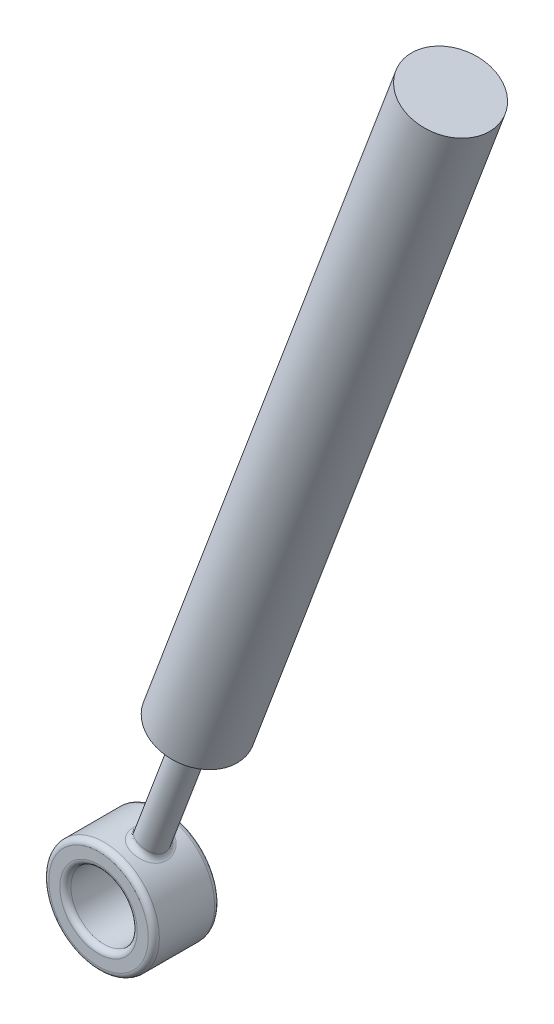
from build123d import *

# Parameters (mm, degrees)
BOSS_EXTRUDE1_START      = -260
BOSS_EXTRUDE1_DEPTH      = 260
BOSS_EXTRUDE4_DEPTH      = 24
BOSS_EXTRUDE5_REACH      = 2447.334
BOSS_EXTRUDE5_END_RADIUS = 20
SKETCH5_R                = 5
FILLET1_R                = 2
FILLET2_R                = 2
CHAMFER2_SIZE            = 1


with BuildPart() as part:
    # Sketch1 → Boss-Extrude1 (new body)
    with BuildSketch(Plane(origin=(83.573308801, 222.892709782, 0), x_dir=(0.9363450005078556, -0.3510812441927706, 0), z_dir=(-0.3510812441927706, -0.9363450005078556, 0)).offset(BOSS_EXTRUDE1_START)):
        with BuildLine():
            ThreePointArc((546.192823225, 2320.014515708), (561.248526003, 2335.070218486), (546.192823225, 2350.125921264))
            ThreePointArc((546.192823225, 2350.125921264), (531.137120447, 2335.070218486), (546.192823225, 2320.014515708))
        make_face()
    extrude(amount=BOSS_EXTRUDE1_DEPTH)



with BuildPart() as body_2:
    # Sketch6 → Boss-Extrude4 (new body)
    with BuildSketch(Plane(origin=(0, 0, 2323.070218486), x_dir=(-1, 0, 0), z_dir=(0, 0, -1))):
        with BuildLine():
            ThreePointArc((-589.676062924, -40.026603584), (-563.92753803, -51.73187871), (-552.222262904, -25.983353816))
            ThreePointArc((-552.222262904, -25.983353816), (-577.970787798, -14.27807869), (-589.676062924, -40.026603584))
        make_face()
        with BuildLine():
            ThreePointArc((-582.18530292, -37.21795363), (-566.736188003, -44.241118713), (-559.713022893, -28.792003808))
            ThreePointArc((-559.713022893, -28.792003808), (-575.162137825, -21.768838687), (-582.18530292, -37.21795363))
        make_face(mode=Mode.SUBTRACT)
    extrude(amount=-BOSS_EXTRUDE4_DEPTH)


with BuildPart() as part_1:
    add(part.part)

    add(body_2.part)  # Boss-Extrude5 merges body 2
    # Boss-Extrude5: up to this cylinder (the profile starts outside it)
    boss_extrude5_end = Plane(origin=(570.949162914, -33.0049787, 2335.070218), z_dir=(0, 0, -1)) * Cylinder(BOSS_EXTRUDE5_END_RADIUS, 4935.668, mode=Mode.PRIVATE)
    # Sketch5 → Boss-Extrude5 (add, up to the surface)
    with BuildSketch(Plane(origin=(83.573308801, 222.892709782, 0), x_dir=(0.9363450005078556, -0.3510812441927706, 0), z_dir=(-0.3510812441927706, -0.9363450005078556, 0)), mode=Mode.PRIVATE) as boss_extrude5_sk1:
        with Locations(Location((546.192823225, 2335.070218486, 0), (0, 0, 180))):
            Circle(SKETCH5_R)
    boss_extrude5_tool1 = extrude(boss_extrude5_sk1.sketch, amount=BOSS_EXTRUDE5_REACH, mode=Mode.PRIVATE) - boss_extrude5_end
    add(boss_extrude5_tool1.solids().sort_by_distance((594.998228, 31.134654, 2335.070218))[0])

    # Fillet1
    fillet1_edges = [part_1.edges().sort_by_distance(p)[0] for p in [
        (582.429546976, -16.628141955, 2335.070218486),
    ]]
    fillet(fillet1_edges, radius=FILLET1_R)

    # Fillet2
    fillet2_edges = [part_1.edges().sort_by_distance(p)[0] for p in [
        (559.713022908, -28.79200377, 2347.070218486),
        (589.676062924, -40.026603584, 2347.070218486),
        (559.713022908, -28.79200377, 2323.070218486),
        (589.676062924, -40.026603584, 2323.070218486),
    ]]
    fillet(fillet2_edges, radius=FILLET2_R)

    # Chamfer2
    chamfer2_edges = [part_1.edges().sort_by_distance(p)[0] for p in [
        (599.679953144, 29.379247614, 2335.070218486),
    ]]
    chamfer(chamfer2_edges, length=CHAMFER2_SIZE)


solid = part_1.part
